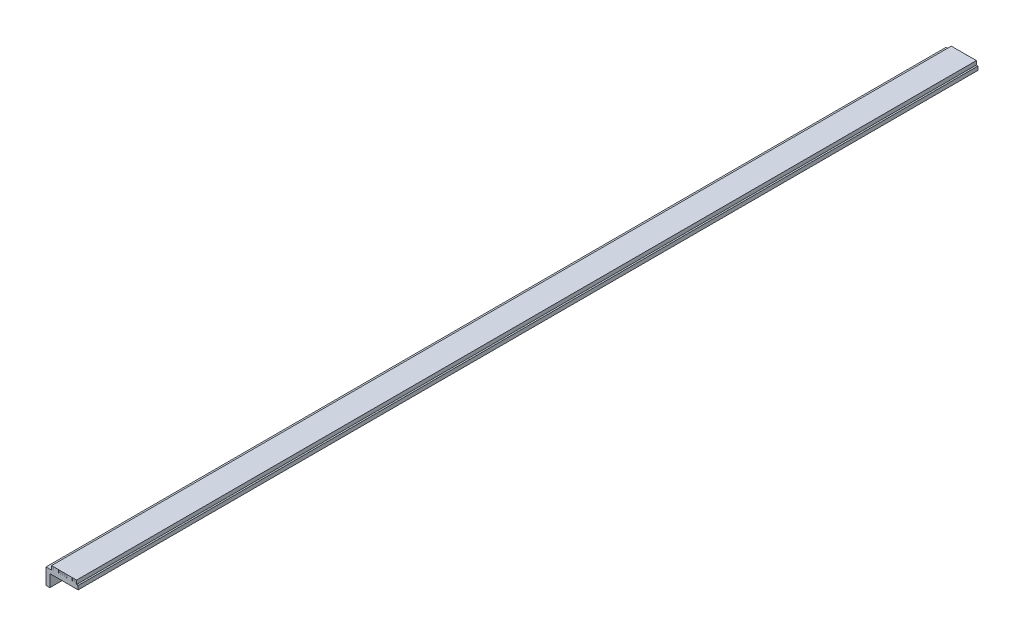
from build123d import *

# Parameters (mm, degrees)
BOSS_EXTRUDE1_DEPTH      = 2800
SKETCH2_W                = 1.259860676
SKETCH2_H                = 9.043092937
CUT_EXTRUDE1_DEPTH       = 0.2
LPATTERN1_COUNT          = 16
LPATTERN1_PITCH          = 6
MIRROR1_COPY_1_SKETCH_W  = 1.259860676
MIRROR1_COPY_1_SKETCH_H  = 9.043092937
MIRROR1_COPY_1_DEPTH     = 0.2
MIRROR1_COPY_2_SKETCH_W  = 1.259860676
MIRROR1_COPY_2_SKETCH_H  = 9.043092937
MIRROR1_COPY_2_DEPTH     = 0.2
MIRROR1_COPY_3_SKETCH_W  = 1.259860676
MIRROR1_COPY_3_SKETCH_H  = 9.043092937
MIRROR1_COPY_3_DEPTH     = 0.2
MIRROR1_COPY_4_SKETCH_W  = 1.259860676
MIRROR1_COPY_4_SKETCH_H  = 9.043092937
MIRROR1_COPY_4_DEPTH     = 0.2
MIRROR1_COPY_5_SKETCH_W  = 1.259860676
MIRROR1_COPY_5_SKETCH_H  = 9.043092937
MIRROR1_COPY_5_DEPTH     = 0.2
MIRROR1_COPY_6_SKETCH_W  = 1.259860676
MIRROR1_COPY_6_SKETCH_H  = 9.043092937
MIRROR1_COPY_6_DEPTH     = 0.2
MIRROR1_COPY_7_SKETCH_W  = 1.259860676
MIRROR1_COPY_7_SKETCH_H  = 9.043092937
MIRROR1_COPY_7_DEPTH     = 0.2
MIRROR1_COPY_8_SKETCH_W  = 1.259860676
MIRROR1_COPY_8_SKETCH_H  = 9.043092937
MIRROR1_COPY_8_DEPTH     = 0.2
MIRROR1_COPY_9_SKETCH_W  = 1.259860676
MIRROR1_COPY_9_SKETCH_H  = 9.043092937
MIRROR1_COPY_9_DEPTH     = 0.2
MIRROR1_COPY_10_SKETCH_W = 1.259860676
MIRROR1_COPY_10_SKETCH_H = 9.043092937
MIRROR1_COPY_10_DEPTH    = 0.2
MIRROR1_COPY_11_SKETCH_W = 1.259860676
MIRROR1_COPY_11_SKETCH_H = 9.043092937
MIRROR1_COPY_11_DEPTH    = 0.2
MIRROR1_COPY_12_SKETCH_W = 1.259860676
MIRROR1_COPY_12_SKETCH_H = 9.043092937
MIRROR1_COPY_12_DEPTH    = 0.2
MIRROR1_COPY_13_SKETCH_W = 1.259860676
MIRROR1_COPY_13_SKETCH_H = 9.043092937
MIRROR1_COPY_13_DEPTH    = 0.2
MIRROR1_COPY_14_SKETCH_W = 1.259860676
MIRROR1_COPY_14_SKETCH_H = 9.043092937
MIRROR1_COPY_14_DEPTH    = 0.2
MIRROR1_COPY_15_SKETCH_W = 1.259860676
MIRROR1_COPY_15_SKETCH_H = 9.043092937
MIRROR1_COPY_15_DEPTH    = 0.2
SKETCH5_W                = 12
SKETCH5_H                = 50
BOSS_EXTRUDE2_DEPTH      = 2800
SKETCH3_W                = 12
SKETCH3_H                = 88
CUT_EXTRUDE3_DEPTH       = 2804.569153775


with BuildPart() as part:
    # Sketch1 → Boss-Extrude1 (new body)
    with BuildSketch(Plane.XY):
        Polygon((0, 0), (100, 0), (100, 12), (95, 12), (95, 24), (17, 24), (17, 12), (12, 12), (12, 100), (0, 100), align=None)
    extrude(amount=BOSS_EXTRUDE1_DEPTH)

    # Sketch2 → Cut-Extrude1 (cut)
    with BuildSketch(Plane.XY.offset(2800)):
        with Locations((22.109179897, 19.478453532)):
            Rectangle(SKETCH2_W, SKETCH2_H)
    cut_extrude1 = extrude(amount=-CUT_EXTRUDE1_DEPTH, mode=Mode.SUBTRACT)

    # LPattern1: Cut-Extrude1 ×16
    with Locations(*[(i * LPATTERN1_PITCH, 0, 0) for i in range(1, LPATTERN1_COUNT)]):
        add(cut_extrude1, mode=Mode.SUBTRACT)

    # Mirror1: Cut-Extrude1 across plane
    add(cut_extrude1.mirror(Plane(origin=(0, 0, 1400), x_dir=(1, 0, 0), z_dir=(0, 0, -1))), mode=Mode.SUBTRACT)

    # Mirror1 copy 1 sketch → Mirror1 copy 1 (cut)
    with BuildSketch(Plane(origin=(6, 0, 0), x_dir=(1, 0, 0), z_dir=(0, 0, -1))):
        with Locations((22.109179897, -19.478453532)):
            Rectangle(MIRROR1_COPY_1_SKETCH_W, MIRROR1_COPY_1_SKETCH_H)
    extrude(amount=-MIRROR1_COPY_1_DEPTH, mode=Mode.SUBTRACT)

    # Mirror1 copy 2 sketch → Mirror1 copy 2 (cut)
    with BuildSketch(Plane(origin=(12, 0, 0), x_dir=(1, 0, 0), z_dir=(0, 0, -1))):
        with Locations((22.109179897, -19.478453532)):
            Rectangle(MIRROR1_COPY_2_SKETCH_W, MIRROR1_COPY_2_SKETCH_H)
    extrude(amount=-MIRROR1_COPY_2_DEPTH, mode=Mode.SUBTRACT)

    # Mirror1 copy 3 sketch → Mirror1 copy 3 (cut)
    with BuildSketch(Plane(origin=(18, 0, 0), x_dir=(1, 0, 0), z_dir=(0, 0, -1))):
        with Locations((22.109179897, -19.478453532)):
            Rectangle(MIRROR1_COPY_3_SKETCH_W, MIRROR1_COPY_3_SKETCH_H)
    extrude(amount=-MIRROR1_COPY_3_DEPTH, mode=Mode.SUBTRACT)

    # Mirror1 copy 4 sketch → Mirror1 copy 4 (cut)
    with BuildSketch(Plane(origin=(24, 0, 0), x_dir=(1, 0, 0), z_dir=(0, 0, -1))):
        with Locations((22.109179897, -19.478453532)):
            Rectangle(MIRROR1_COPY_4_SKETCH_W, MIRROR1_COPY_4_SKETCH_H)
    extrude(amount=-MIRROR1_COPY_4_DEPTH, mode=Mode.SUBTRACT)

    # Mirror1 copy 5 sketch → Mirror1 copy 5 (cut)
    with BuildSketch(Plane(origin=(30, 0, 0), x_dir=(1, 0, 0), z_dir=(0, 0, -1))):
        with Locations((22.109179897, -19.478453532)):
            Rectangle(MIRROR1_COPY_5_SKETCH_W, MIRROR1_COPY_5_SKETCH_H)
    extrude(amount=-MIRROR1_COPY_5_DEPTH, mode=Mode.SUBTRACT)

    # Mirror1 copy 6 sketch → Mirror1 copy 6 (cut)
    with BuildSketch(Plane(origin=(36, 0, 0), x_dir=(1, 0, 0), z_dir=(0, 0, -1))):
        with Locations((22.109179897, -19.478453532)):
            Rectangle(MIRROR1_COPY_6_SKETCH_W, MIRROR1_COPY_6_SKETCH_H)
    extrude(amount=-MIRROR1_COPY_6_DEPTH, mode=Mode.SUBTRACT)

    # Mirror1 copy 7 sketch → Mirror1 copy 7 (cut)
    with BuildSketch(Plane(origin=(42, 0, 0), x_dir=(1, 0, 0), z_dir=(0, 0, -1))):
        with Locations((22.109179897, -19.478453532)):
            Rectangle(MIRROR1_COPY_7_SKETCH_W, MIRROR1_COPY_7_SKETCH_H)
    extrude(amount=-MIRROR1_COPY_7_DEPTH, mode=Mode.SUBTRACT)

    # Mirror1 copy 8 sketch → Mirror1 copy 8 (cut)
    with BuildSketch(Plane(origin=(48, 0, 0), x_dir=(1, 0, 0), z_dir=(0, 0, -1))):
        with Locations((22.109179897, -19.478453532)):
            Rectangle(MIRROR1_COPY_8_SKETCH_W, MIRROR1_COPY_8_SKETCH_H)
    extrude(amount=-MIRROR1_COPY_8_DEPTH, mode=Mode.SUBTRACT)

    # Mirror1 copy 9 sketch → Mirror1 copy 9 (cut)
    with BuildSketch(Plane(origin=(54, 0, 0), x_dir=(1, 0, 0), z_dir=(0, 0, -1))):
        with Locations((22.109179897, -19.478453532)):
            Rectangle(MIRROR1_COPY_9_SKETCH_W, MIRROR1_COPY_9_SKETCH_H)
    extrude(amount=-MIRROR1_COPY_9_DEPTH, mode=Mode.SUBTRACT)

    # Mirror1 copy 10 sketch → Mirror1 copy 10 (cut)
    with BuildSketch(Plane(origin=(60, 0, 0), x_dir=(1, 0, 0), z_dir=(0, 0, -1))):
        with Locations((22.109179897, -19.478453532)):
            Rectangle(MIRROR1_COPY_10_SKETCH_W, MIRROR1_COPY_10_SKETCH_H)
    extrude(amount=-MIRROR1_COPY_10_DEPTH, mode=Mode.SUBTRACT)

    # Mirror1 copy 11 sketch → Mirror1 copy 11 (cut)
    with BuildSketch(Plane(origin=(66, 0, 0), x_dir=(1, 0, 0), z_dir=(0, 0, -1))):
        with Locations((22.109179897, -19.478453532)):
            Rectangle(MIRROR1_COPY_11_SKETCH_W, MIRROR1_COPY_11_SKETCH_H)
    extrude(amount=-MIRROR1_COPY_11_DEPTH, mode=Mode.SUBTRACT)

    # Mirror1 copy 12 sketch → Mirror1 copy 12 (cut)
    with BuildSketch(Plane(origin=(72, 0, 0), x_dir=(1, 0, 0), z_dir=(0, 0, -1))):
        with Locations((22.109179897, -19.478453532)):
            Rectangle(MIRROR1_COPY_12_SKETCH_W, MIRROR1_COPY_12_SKETCH_H)
    extrude(amount=-MIRROR1_COPY_12_DEPTH, mode=Mode.SUBTRACT)

    # Mirror1 copy 13 sketch → Mirror1 copy 13 (cut)
    with BuildSketch(Plane(origin=(78, 0, 0), x_dir=(1, 0, 0), z_dir=(0, 0, -1))):
        with Locations((22.109179897, -19.478453532)):
            Rectangle(MIRROR1_COPY_13_SKETCH_W, MIRROR1_COPY_13_SKETCH_H)
    extrude(amount=-MIRROR1_COPY_13_DEPTH, mode=Mode.SUBTRACT)

    # Mirror1 copy 14 sketch → Mirror1 copy 14 (cut)
    with BuildSketch(Plane(origin=(84, 0, 0), x_dir=(1, 0, 0), z_dir=(0, 0, -1))):
        with Locations((22.109179897, -19.478453532)):
            Rectangle(MIRROR1_COPY_14_SKETCH_W, MIRROR1_COPY_14_SKETCH_H)
    extrude(amount=-MIRROR1_COPY_14_DEPTH, mode=Mode.SUBTRACT)

    # Mirror1 copy 15 sketch → Mirror1 copy 15 (cut)
    with BuildSketch(Plane(origin=(90, 0, 0), x_dir=(1, 0, 0), z_dir=(0, 0, -1))):
        with Locations((22.109179897, -19.478453532)):
            Rectangle(MIRROR1_COPY_15_SKETCH_W, MIRROR1_COPY_15_SKETCH_H)
    extrude(amount=-MIRROR1_COPY_15_DEPTH, mode=Mode.SUBTRACT)

    # Sketch5 → Boss-Extrude2 (add)
    with BuildSketch(Plane.XY.offset(2800)):
        with Locations((6, -13)):
            Rectangle(SKETCH5_W, SKETCH5_H)
    extrude(amount=-BOSS_EXTRUDE2_DEPTH)

    # Sketch3 → Cut-Extrude3 (cut, through all)
    with BuildSketch(Plane.XY.offset(2800)):
        with Locations((6, 56)):
            Rectangle(SKETCH3_W, SKETCH3_H)
    extrude(amount=-CUT_EXTRUDE3_DEPTH, mode=Mode.SUBTRACT)


solid = part.part
